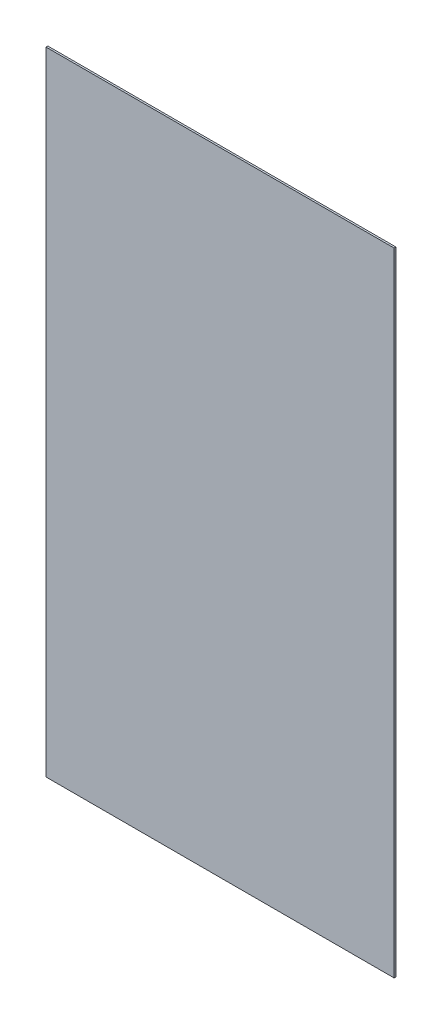
SolidWorks part; units mm, degrees
ref_plane "前视基准面" through (0, 0, 0) normal (0, 0, 1) x (1, 0, 0)
ref_plane "上视基准面" through (0, 0, 0) normal (0, 1, 0) x (1, 0, 0)
ref_plane "右视基准面" through (0, 0, 0) normal (1, 0, 0) x (0, 0, -1)
sketch "草图1" plane through (0, 0, 0) normal (0, 0, 1) x (1, 0, 0)
  line L1 (-337.8818, 161.4532) -> (42.1182, 161.4532)
  line L2 (-337.8818, 161.4532) -> (-337.8818, -528.5468)
  line L3 (-337.8818, -528.5468) -> (42.1182, -528.5468)
  line L4 (42.1182, 161.4532) -> (42.1182, -528.5468)
  dimension "D1" = 690
  dimension "D2" = 380
extrude "凸台-拉伸1" add sketch "草图1" along normal blind 2
